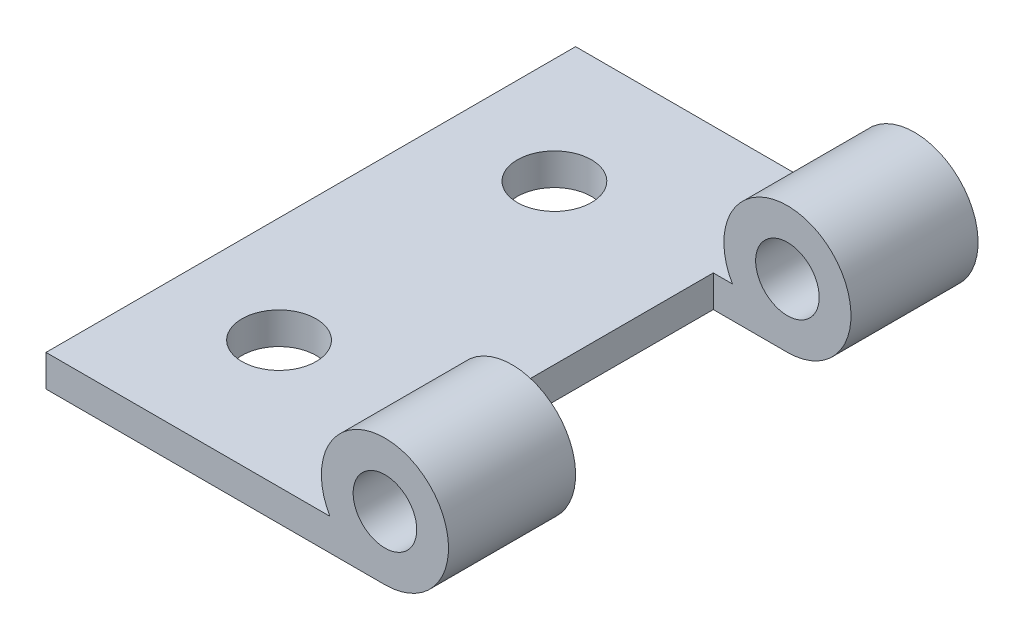
SolidWorks part; units mm, degrees
material "AISI 304"
ref_plane "前视基准面" through (0, 0, 0) normal (0, 0, 1) x (1, 0, 0)
ref_plane "上视基准面" through (0, 0, 0) normal (0, 1, 0) x (1, 0, 0)
ref_plane "右视基准面" through (0, 0, 0) normal (1, 0, 0) x (0, 0, -1)
sketch "草图1" plane through (0, 0, 0) normal (0, 0, 1) x (1, 0, 0)
  line L0 (-2.5981, -1.5) -> (-16, -1.5)
  line L1 (-16, -1.5) -> (-16, -3)
  line L2 (-16, -3) -> (0, -3)
  circle A0 centre (0, 0) radius 1.5
  arc A1 (0, -3) -> (-2.5981, -1.5) centre (0, 0) ccw
  dimension "D1" = 6
  dimension "D2" = 3
  dimension "D3" = 16
extrude "凸台-拉伸1" add sketch "草图1" along normal mid plane 25
sketch "草图2" plane through (0, 0, 0) normal (0, 0, 1) x (1, 0, 0)
  line L0 (-3.5, 0) -> (-3.5, -3)
  line L1 (-16, -3) -> (0, -3) construction
  line L3 (-3.5, -3) -> (-1.8028, -3)
  arc A0 (-1.8028, -3) -> (-3.5, 0) centre (0, 0) ccw
  dimension "D1" = 3.5
extrude "切除-拉伸1" cut sketch "草图2" against normal mid plane 13
sketch "草图3" plane through (0, -1.5, 0) normal (0, 1, 0) x (1, 0, 0)
  line L0 (0, 0) -> (-16, 0) construction
  line L1 (-16, -12.5) -> (-16, 12.5) construction
  circle A0 centre (-11, 6.5) radius 1.75
  circle A1 centre (-11, -6.5) radius 1.75
  dimension "D1" = 3.5
  dimension "D2" = 11
  dimension "D3" = 13
extrude "切除-拉伸2" cut sketch "草图3" against normal through all
